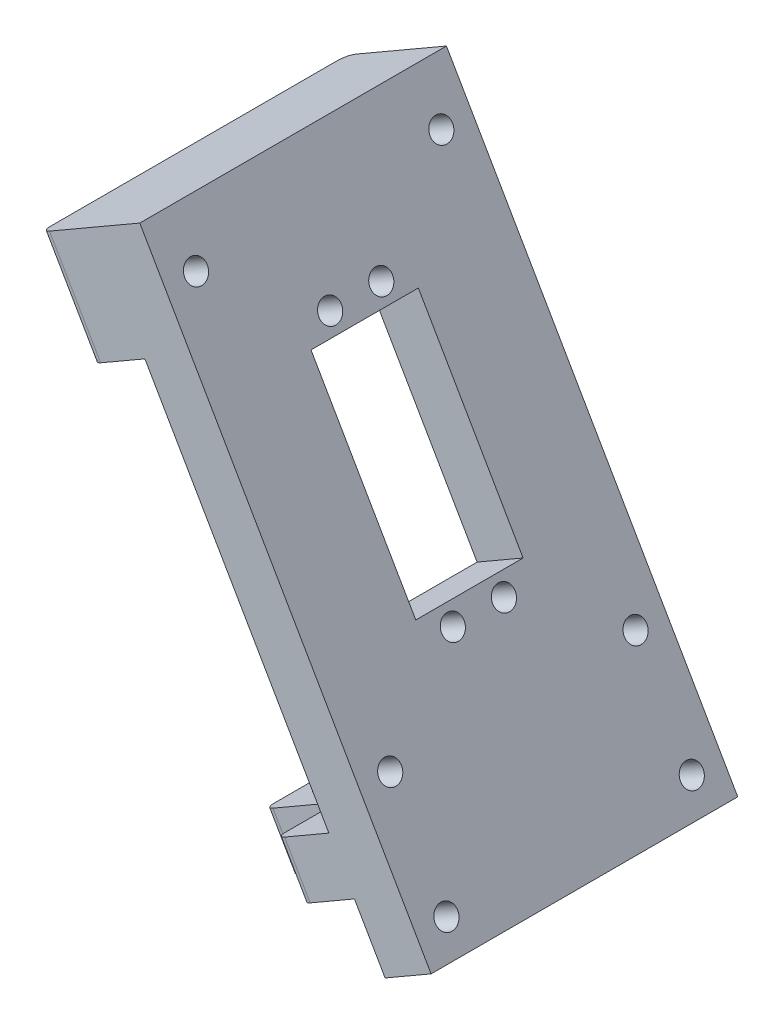
from build123d import *

# Parameters (mm, degrees)
SKETCH_1_W          = 12
SKETCH_1_H          = 26
EXTRUDE_1_DEPTH     = 30
EXTRUDE_2_DEPTH     = 60
SKETCH_3_W          = 60
SKETCH_3_H          = 20
EXTRUDE_3_DEPTH     = 12
EXTRUDE_START       = 72
SKETCH_5_W          = 26
SKETCH_5_H          = 11.5
EXTRUDE_4_DEPTH     = 10
SKETCH_6_W          = 21
SKETCH_6_H          = 41
CUT_EXTRUDE_1_DEPTH = 55
SKETCH_7_R          = 2.2
CUT_EXTRUDE_2_DEPTH = 41
FILLET_1_R          = 20
SKETCH_8_R          = 3.3
CUT_EXTRUDE_3_DEPTH = 21
FILLET_2_R          = 2
FILLET_3_R          = 2
FILLET_4_R          = 2
SKETCH_9_W          = 60
SKETCH_9_H          = 60.516660498
CUT_EXTRUDE_4_DEPTH = 35
SKETCH_10_R         = 2.2
CUT_EXTRUDE_5_DEPTH = 71
SKETCH_12_R         = 2.2
CUT_EXTRUDE_6_DEPTH = 113


with BuildPart() as part:
    # 草图1 → 凸台-拉伸1 (new, symmetric)
    with BuildSketch(Plane.XY):
        Rectangle(SKETCH_1_W, SKETCH_1_H)
    extrude(amount=EXTRUDE_1_DEPTH, both=True)

    # 草图2 → 凸台-拉伸2 (add)
    with BuildSketch(Plane(origin=(0, 0, -30), x_dir=(-1, 0, 0), z_dir=(0, 0, -1))):
        Polygon((6, 13), (71, 125.583302492), (62, 130.779454915), (-6, 13), align=None)
    extrude(amount=-EXTRUDE_2_DEPTH)

    # 草图3 → 凸台-拉伸3 (add)
    with BuildSketch(Plane(origin=(1.129165125, 0.651923789, 0), x_dir=(0, 0, 1), z_dir=(-0.866025403784438, -0.500000000000001, 0))):
        with Locations((0, 134.258330249)):
            Rectangle(SKETCH_3_W, SKETCH_3_H)
    extrude(amount=EXTRUDE_3_DEPTH)

    # 草图5 → 凸台-拉伸4 (add)
    with BuildSketch(Plane(origin=(-62.129165125, 107.610870628, 0), x_dir=(0, 0, -1), z_dir=(0.500000000000001, -0.866025403784438, 0)).offset(EXTRUDE_START)):
        Polygon((30, -10.696152423), (30, 1.303847577), (-30, 1.303847577), (-30, -10.696152423), (-18, -10.696152423), (-18, -27.196152423), (18, -27.196152423), (18, -10.696152423), align=None)
        with Locations((0, -16.446152423)):
            Rectangle(SKETCH_5_W, SKETCH_5_H, mode=Mode.SUBTRACT)
    extrude(amount=EXTRUDE_4_DEPTH)

    # 草图6 → 切除-拉伸1 (cut)
    with BuildSketch(Plane(origin=(10.129165125, 5.848076211, 0), x_dir=(0, 0, -1), z_dir=(0.8660254037844382, 0.500000000000001, 0))):
        with Locations((0, 95.758330249)):
            Rectangle(SKETCH_6_W, SKETCH_6_H)
    extrude(amount=-CUT_EXTRUDE_1_DEPTH, mode=Mode.SUBTRACT)

    # 草图7 → 切除-拉伸2 (cut)
    with BuildSketch(Plane(origin=(10.129165125, 5.848076211, 0), x_dir=(0, 0, -1), z_dir=(0.8660254037844382, 0.500000000000001, 0))):
        with Locations(Location((5, 71.758330249, 0), (0, 0, 90))):
            Circle(SKETCH_7_R)
        with Locations(Location((-5, 71.758330249, 0), (0, 0, 90))):
            Circle(SKETCH_7_R)
        with Locations(Location((5, 119.758330249, 0), (0, 0, 90))):
            Circle(SKETCH_7_R)
        with Locations(Location((-5, 119.758330249, 0), (0, 0, 90))):
            Circle(SKETCH_7_R)
    extrude(amount=-CUT_EXTRUDE_2_DEPTH, mode=Mode.SUBTRACT)

    # 圆角1
    fillet_1_edges = [part.edges().sort_by_distance(p)[0] for p in [
        (-6, 13, 0),
        (6, 13, 0),
    ]]
    fillet(fillet_1_edges, radius=FILLET_1_R)

    # 草图8 → 切除-拉伸3 (cut)
    with BuildSketch(Plane.ZY.offset(6)):
        with Locations((-12.5, -3)):
            Circle(SKETCH_8_R)
        with Locations((12.5, -3)):
            Circle(SKETCH_8_R)
    extrude(amount=-CUT_EXTRUDE_3_DEPTH, mode=Mode.SUBTRACT)

    # 圆角2
    fillet_2_edges = [part.edges().sort_by_distance(p)[0] for p in [
        (0, -13, 30),
        (0, -13, -30),
    ]]
    fillet(fillet_2_edges, radius=FILLET_2_R)

    # 圆角3
    fillet_3_edges = [part.edges().sort_by_distance(p)[0] for p in [
        (-32.892304845, 35.578838325, -30),
        (-32.892304845, 35.578838325, 30),
        (-32.892304845, 35.578838325, 18),
        (-47.181724008, 27.328838325, 18),
        (-47.181724008, 27.328838325, -18),
        (-32.892304845, 35.578838325, -18),
    ]]
    fillet(fillet_3_edges, radius=FILLET_3_R)

    # 圆角4
    fillet_4_edges = [part.edges().sort_by_distance(p)[0] for p in [
        (-76.392304845, 110.923048454, 30),
        (-76.392304845, 110.923048454, -30),
    ]]
    fillet(fillet_4_edges, radius=FILLET_4_R)

    # 草图9 → 切除-拉伸4 (cut, symmetric)
    with BuildSketch(Plane(origin=(1.129165125, 0.651923789, 0), x_dir=(0, 0, 1), z_dir=(-0.8660254037844382, -0.500000000000001, 0))):
        Rectangle(SKETCH_9_W, SKETCH_9_H)
    extrude(amount=CUT_EXTRUDE_4_DEPTH, both=True, mode=Mode.SUBTRACT)

    # 草图10 → 切除-拉伸5 (cut)
    with BuildSketch(Plane(origin=(-9.263139721, -5.348076211, 0), x_dir=(0, 0, 1), z_dir=(-0.866025403784438, -0.5000000000000009, 0))):
        with Locations(Location((24, 134.258330249, 0), (0, 0, 270))):
            Circle(SKETCH_10_R)
        with Locations(Location((-24, 134.258330249, 0), (0, 0, 270))):
            Circle(SKETCH_10_R)
    extrude(amount=-CUT_EXTRUDE_5_DEPTH, mode=Mode.SUBTRACT)

    # 草图12 → 切除-拉伸6 (cut)
    with BuildSketch(Plane(origin=(1.129165125, 0.651923789, 0), x_dir=(0, 0, 1), z_dir=(-0.8660254037844382, -0.500000000000001, 0))):
        with Locations(Location((-24, 58.258330249, 0), (0, 0, 270))):
            Circle(SKETCH_12_R)
        with Locations(Location((24, 58.258330249, 0), (0, 0, 270))):
            Circle(SKETCH_12_R)
        with Locations(Location((24, 36.258330249, 0), (0, 0, 270))):
            Circle(SKETCH_12_R)
        with Locations(Location((-24, 36.258330249, 0), (0, 0, 270))):
            Circle(SKETCH_12_R)
    extrude(amount=-CUT_EXTRUDE_6_DEPTH, mode=Mode.SUBTRACT)


solid = part.part
